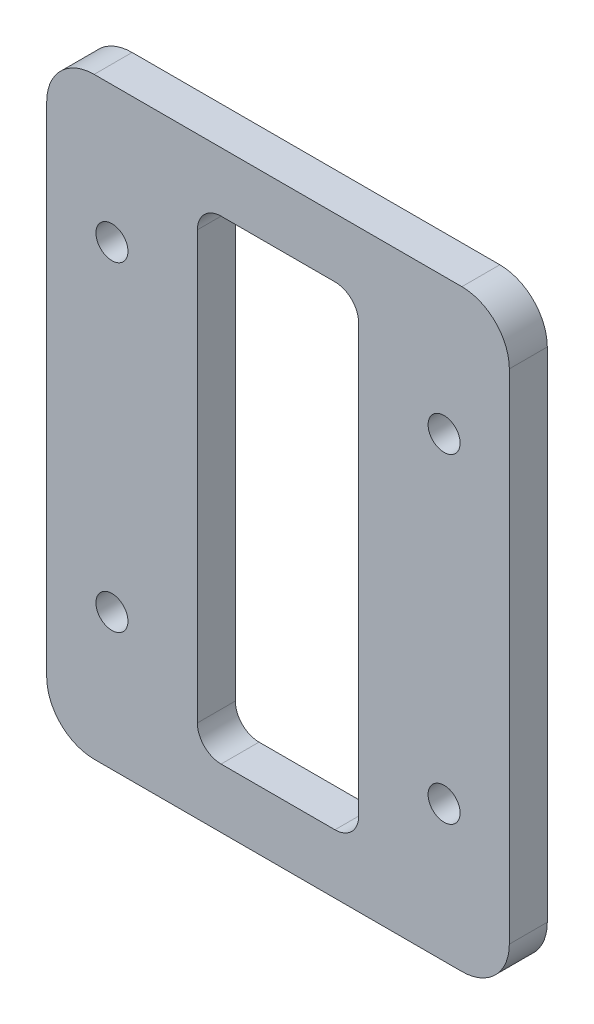
SolidWorks part; units mm, degrees
material "Q235B"
ref_plane "Front Plane" through (0, 0, 0) normal (0, 0, 1) x (1, 0, 0)
ref_plane "Top Plane" through (0, 0, 0) normal (0, 1, 0) x (1, 0, 0)
ref_plane "Right Plane" through (0, 0, 0) normal (1, 0, 0) x (0, 0, -1)
sketch "Sketch1" plane through (0, 0, 0) normal (0, 0, 1) x (1, 0, 0)
  line L1 (97.5, -125) -> (-97.5, -125)
  line L2 (97.5, -125) -> (97.5, 125)
  line L3 (97.5, 125) -> (-97.5, 125)
  line L4 (-97.5, -125) -> (-97.5, 125)
  line L5 (97.5, -125) -> (-97.5, 125) construction
  line L6 (97.5, 125) -> (-97.5, -125) construction
  line L7 (34, -100) -> (-34, -100)
  line L8 (34, -100) -> (34, 100)
  line L9 (34, 100) -> (-34, 100)
  line L10 (-34, -100) -> (-34, 100)
  line L11 (34, -100) -> (-34, 100) construction
  line L12 (34, 100) -> (-34, -100) construction
  point P0 (0, 0)
  point P5 (0, 0)
  dimension "D1" = 250
  dimension "D2" = 195
  dimension "D3" = 200
  dimension "D4" = 68
extrude "Boss-Extrude1" add sketch "Sketch1" along normal mid plane 16
hole_wizard "Ø13.5 Hole1" positions "Sketch2" profile "Sketch3" hole size "Ø18.0" standard "GB" end condition up to next
sketch "Sketch2" plane through (0, 0, 8) normal (0, 0, 1) x (1, 0, 0)
  line L0 (0, 125) -> (0, 0) construction
  line L1 (97.5, 125) -> (-97.5, 125) construction
  line L2 (0, 0) -> (-97.5, 0) construction
  line L3 (-97.5, 125) -> (-97.5, -125) construction
  point P0 (-70, 67.5)
  point P13 (70, 67.5)
  point P14 (70, -67.5)
  point P15 (-70, -67.5)
  dimension "D1" = 140
  dimension "D2" = 135
sketch "Sketch3" plane through (-70, 67.5, 8) normal (1, 0, 0) x (0, -1, 0)
  line L0 (0, 0) -> (0, 16)
  line L1 (0, 16) -> (6.75, 16)
  line L2 (6.75, 16) -> (6.75, 0)
  line L5 (6.75, 0) -> (0, 0)
  line L11 (0, -6.35) -> (0, 107.95) construction
  dimension "通孔孔直径" = 13.5
  dimension "通孔孔深度" = 16
chamfer "Chamfer1" [suppressed] distance 10 angle 45
fillet "Fillet2" radius 20 4 edges at (97.5, 125, 0) (97.5, -125, 0) (-97.5, -125, 0) (-97.5, 125, 0)
fillet "Fillet3" radius 10 4 edges at (34, 100, 0) (-34, 100, 0) (34, -100, 0) (-34, -100, 0)
